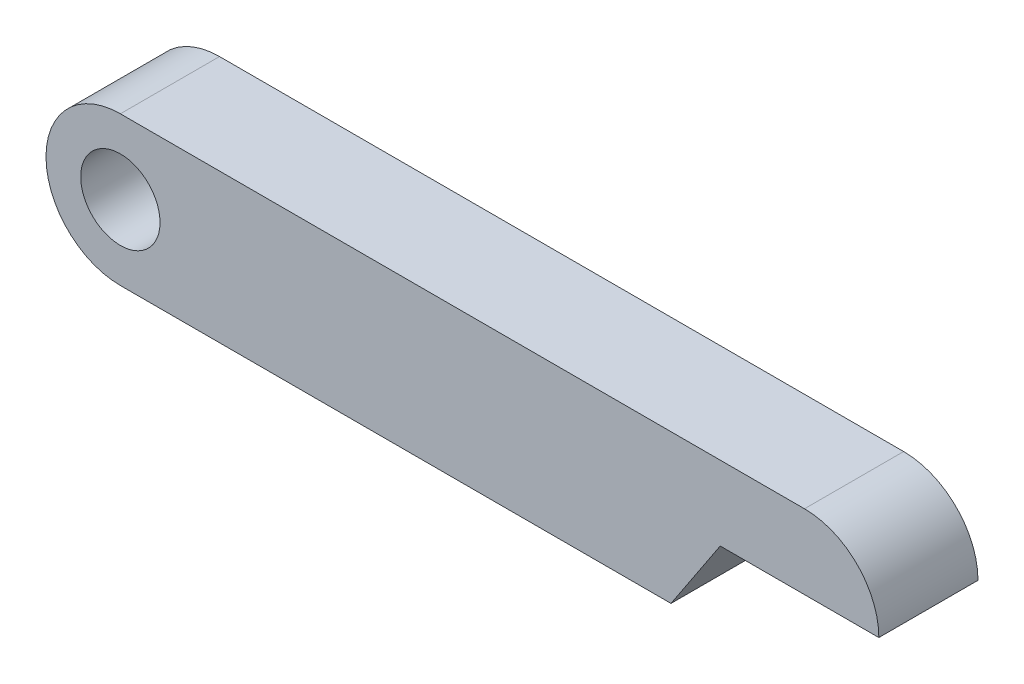
SolidWorks part; units mm, degrees
ref_plane "Front Plane" through (0, 0, 0) normal (0, 0, 1) x (1, 0, 0)
ref_plane "Top Plane" through (0, 0, 0) normal (0, 1, 0) x (1, 0, 0)
ref_plane "Right Plane" through (0, 0, 0) normal (1, 0, 0) x (0, 0, -1)
sketch "Sketch1" plane through (0, 0, 0) normal (0, 0, 1) x (1, 0, 0)
  line L0 (0, 7.5) -> (69, 7.5)
  line L1 (55.5356, -7.5) -> (0, -7.5)
  line L2 (55.5356, -7.5) -> (60.5, 0)
  line L3 (60.5, 0) -> (76.5, 0)
  circle A0 centre (0, 0) radius 4
  arc A2 (0, 7.5) -> (0, -7.5) centre (0, 0) ccw
  arc A3 (76.5, 0) -> (69, 7.5) centre (69, 0) ccw
  dimension "D1" = 69
  dimension "D2" = 8
  dimension "D3" = 15
  dimension "D4" = 16
extrude "Boss-Extrude1" add sketch "Sketch1" along normal blind 10
